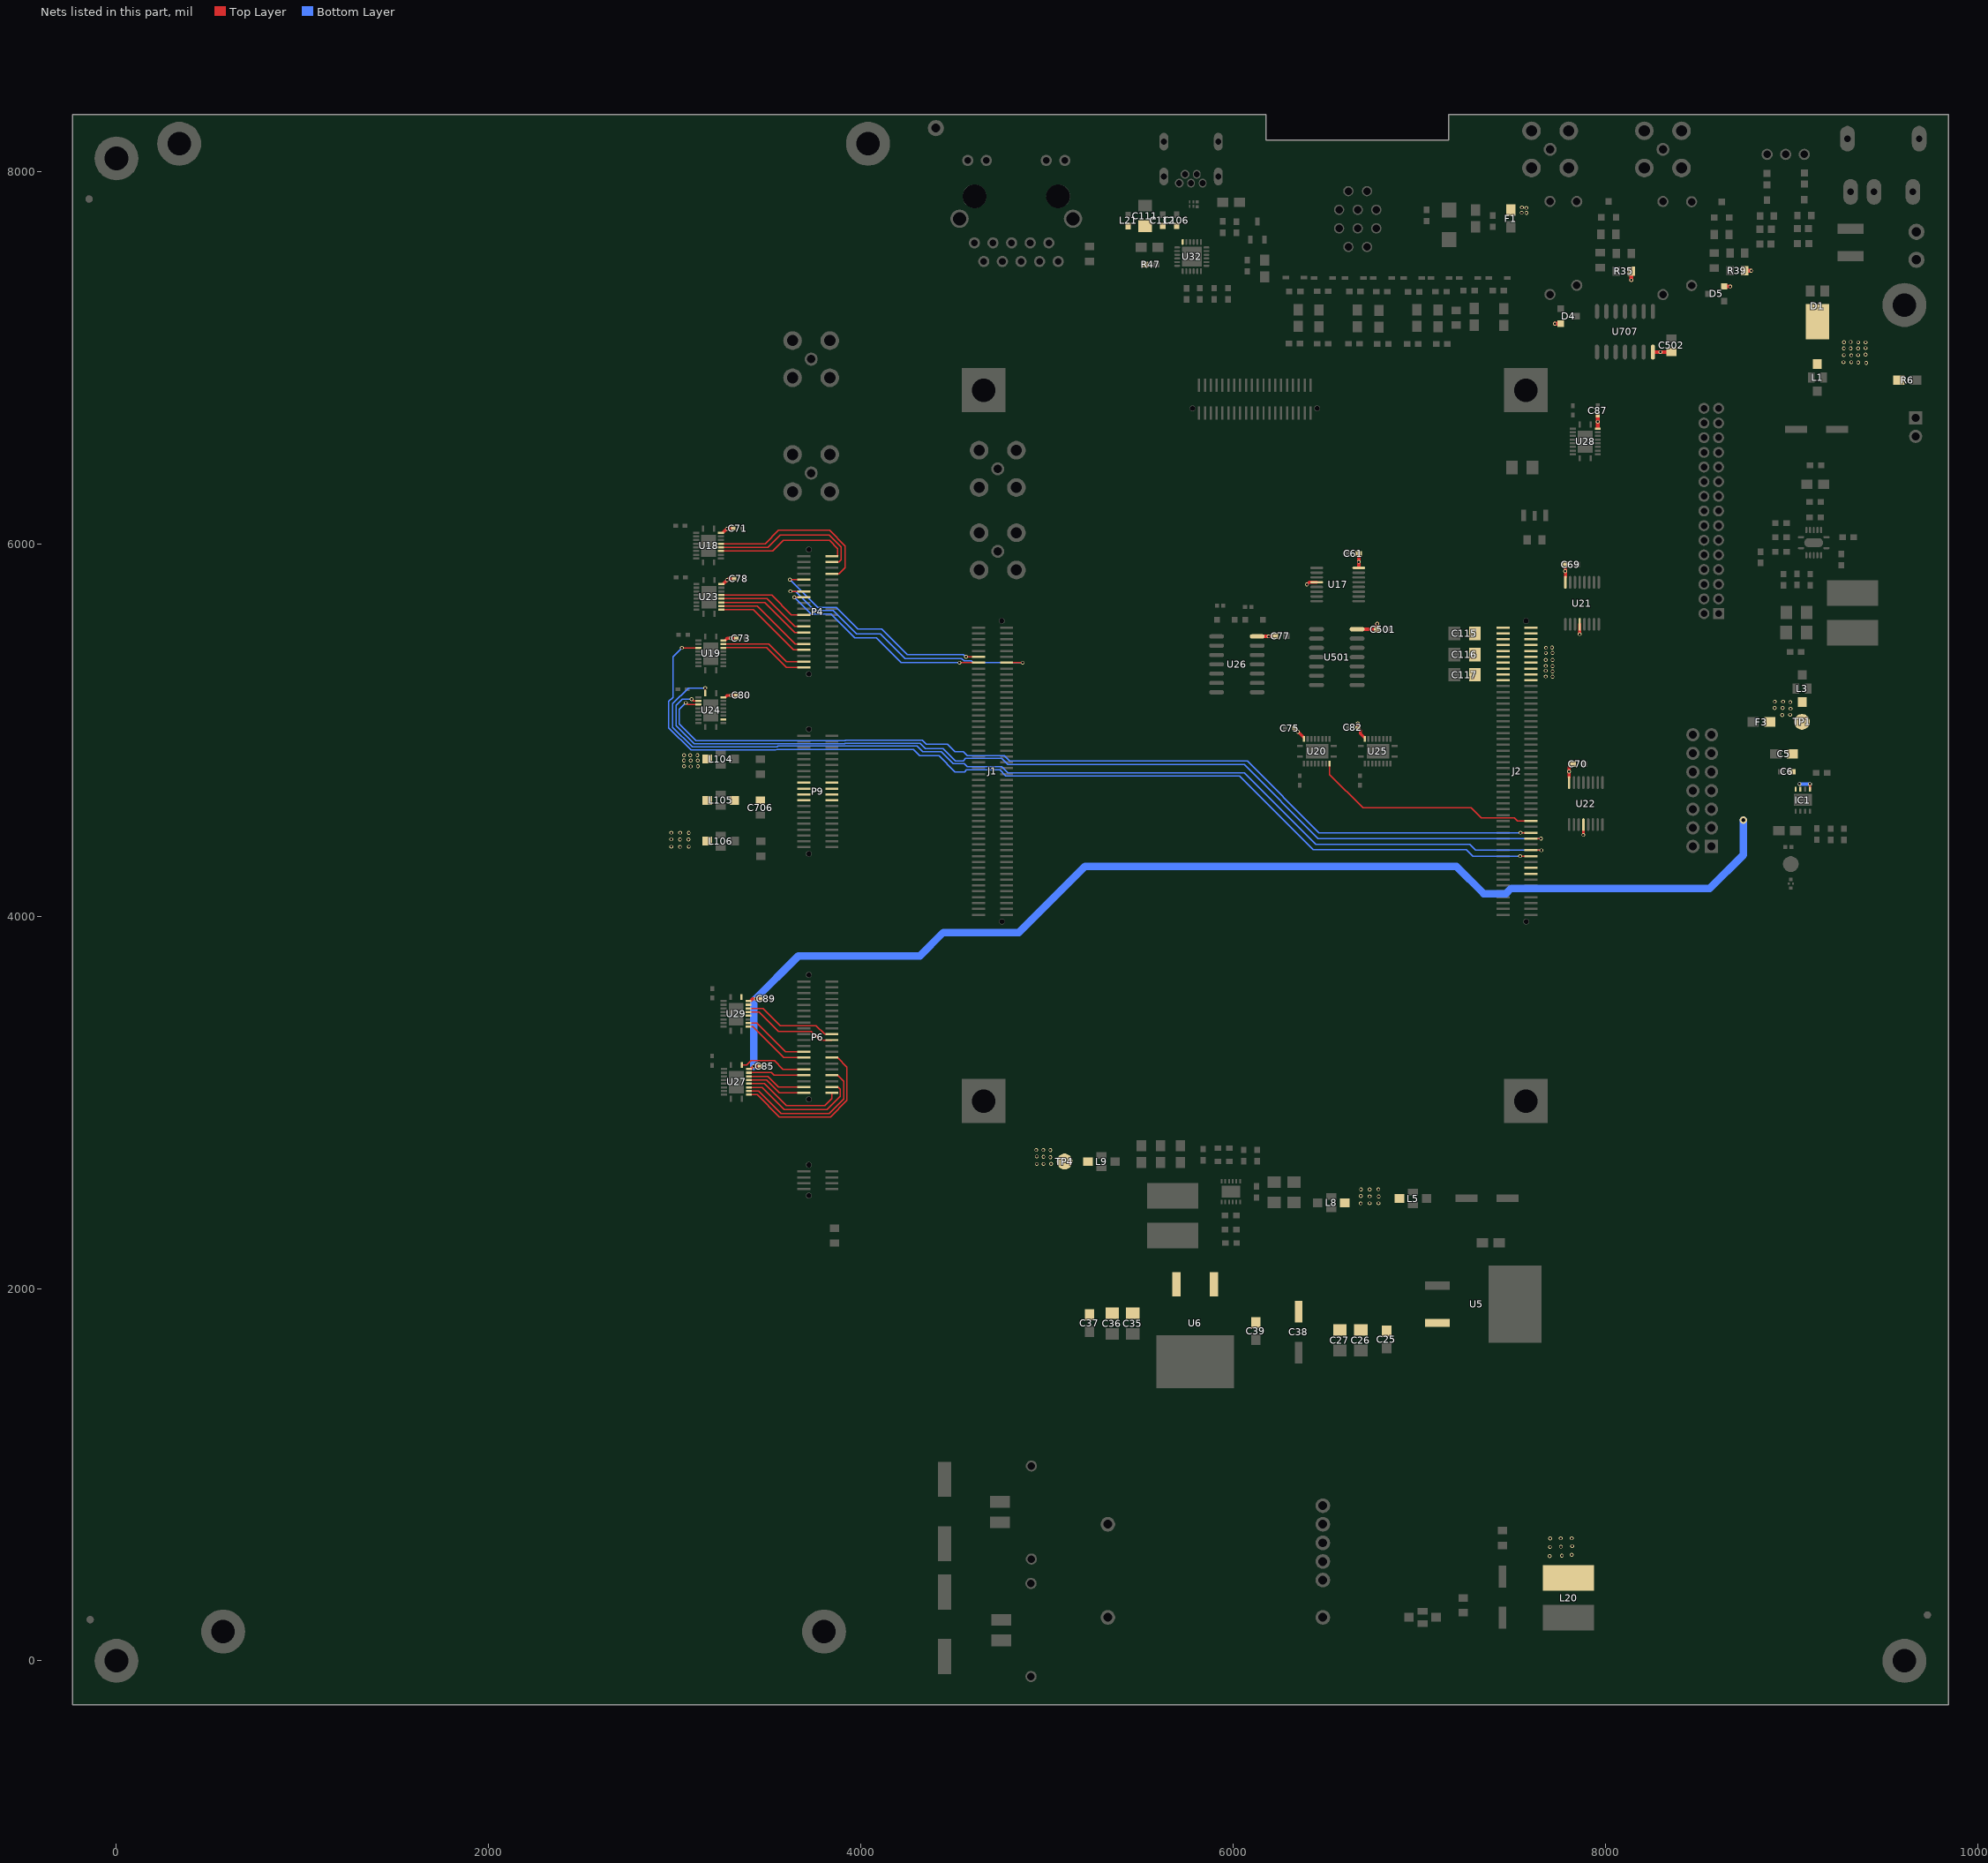
[diagram p0: the nets of this part, all layers, seen from the top]
# Altium PCB MISC82191.PcbDoc (part 4 of 9)
Units mil, origin at the board's own origin, x right, y up, seen from the top; angles counter-clockwise.
Board outline 10078.74 x 8543.31 mil, 4 copper layers (Top Layer, GND, POWER, Bottom Layer); 238 components, 299 nets, 1297 pads, 1665 vias.

## Via types
v1: diameter 20, hole 12, Top Layer to Bottom Layer, 1664 vias
v2: diameter 40, hole 20, Top Layer to Bottom Layer, 1 vias

## Nets (pads, with @x,y where several pads share a name; then routed paths per layer and width w, separated by ;. In a path a pad name is that pad's centre, name@x,y a point inside that pad or via, vN(x,y) a via of type N, cw(c..) or ccw(c..) an arc to the next point about the centre after c; other vN are vias at no path point) (continued)
3VIO58: J2.A34 U20.9 | length 1242
  Top Layer w6: U20.9@6518.25,4819.32 6518.25,4761.68 6697.78,4582.16 7277.78,4582.16 7331.78,4528.16 7509.78,4528.16 7526.3,4511.64 J2.A34@7599.01,4511.64
3VIO60: J2.A37 U24.3 | length 5298.9
  Top Layer w6: v1(3089.78,5166.16) 3099.5,5156.44 U24.3@3126.38,5156.44 ; J2.A37@7599.01,4417.15 v1(7653.79,4417.15)
  Bottom Layer w6: v1(3089.78,5166.16) 3040.78,5166.16 3007.78,5133.16 3007.78,5024.16 3104.53,4927.41 3912.03,4927.41 3913.78,4929.16 ; 3921.78,4929.16 3913.78,4929.16 ; 4907.78,4814.16 4900.78,4814.16 ; 7627.78,4417.16 7551.78,4417.16 ; v1@7652.78,4417.16 7551.78,4417.16 ; 3913.78,4929.16 4317.78,4929.16 4345.78,4901.16 4440.78,4901.16 4506.78,4835.16 4549.78,4835.16 4561.78,4847.16 4756.78,4847.16 4789.78,4814.16 4900.78,4814.16 ; 4900.78,4814.16 6059.03,4814.16 6456.03,4417.16 7551.78,4417.16
3VIO61: J2.A40 U19.4 | length 5542.8
  Top Layer w6: v1(3038.18,5441.76) U19.4@3126.38,5441.76 ; v1(7541.28,4322.66) J2.A40@7599.01,4322.66
  Bottom Layer w6: v1(3038.18,5441.76) 2989.78,5393.35 2989.78,5176.16 2966.78,5153.16 2966.78,5012.16 3086.53,4892.41 3543.03,4892.41 3546.78,4896.16 ; 3561.78,4896.16 3546.78,4896.16 ; 3881.53,4895.41 4282.78,4895.41 4316.03,4862.16 4342.78,4862.16 ; 3881.53,4896.16 3546.78,4896.16 ; 4320.78,4862.16 4342.78,4862.16 ; 4920.78,4753.16 4908.78,4753.16 ; 7518.78,4322.16 7499.78,4322.16 ; v1@7538.78,4322.16 7499.78,4322.16 ; 4342.78,4862.16 4418.78,4862.16 4505.78,4775.16 4556.78,4775.16 4567.78,4786.16 4745.78,4786.16 4778.78,4753.16 4908.78,4753.16 ; 4908.78,4753.16 6034.03,4753.16 6430.03,4357.16 7252.03,4357.16 7287.03,4322.16 7499.78,4322.16
3VIO62: J2.A39 U24.1 | length 5480.7
  Top Layer w6: U24.1@3163.78,5197.78 v1(3163.78,5226.16) ; J2.A39@7599.01,4354.16 v1(7655.78,4354.16)
  Bottom Layer w6: v1(3163.78,5226.16) 3073.78,5226.16 2988.78,5141.16 2988.78,5014.16 3093.53,4909.41 3549.03,4909.41 3553.78,4914.16 ; 3561.78,4914.16 3553.78,4914.16 ; 4920.78,4771.16 4911.78,4771.16 ; 7636.78,4355.16 7540.78,4355.16 ; v1@7656.78,4354.16 7655.78,4355.16 7540.78,4355.16 ; 3553.78,4914.16 4301.78,4914.16 4332.78,4883.16 4431.78,4883.16 4495.78,4819.16 4555.78,4819.16 4570.78,4804.16 4756.78,4804.16 4789.78,4771.16 4911.78,4771.16 ; 4911.78,4771.16 6060.03,4771.16 6444.03,4387.16 7271.03,4387.16 7303.03,4355.16 7540.78,4355.16
3VIO63: J2.A42
3VIO64: J2.A43
"9V 1.5A": C25.2 C26.2 C27.2 C38.1 C39.2 U5.3 U6.1
13V: C115.1 C116.2 C117.2 D1.3 J2.A1 J2.A2 J2.A3 J2.A4 J2.A5 J2.A6 J2.A7 J2.A8 J2.A9 J2.A10 J2.B1 J2.B2 J2.B3 J2.B4 J2.B5 J2.B6 J2.B7 J2.B8 J2.B9 J2.B10 L1.1 L5.1 L8.3 L20.1 L106.3 R6.1
  other v1: 7700.78,562.41 7765.78,565.41 7818.78,569.41 7701.78,611.41 7760.78,613.41 7820.78,616.41 7702.78,657.41 7759.78,658.41 7818.78,658.41 6684.78,2457.41 6732.78,2458.41 6780.78,2458.41 6781.78,2494.41 6732.78,2495.41 6685.78,2496.41 6686.78,2532.41 6732.78,2532.41 6779.78,2533.41 3027.78,4372.41 2980.78,4373.41 3074.78,4373.41 3027.78,4412.41 3073.78,4412.41 2980.78,4413.41 3074.78,4447.41 2980.78,4448.41 3028.78,4448.41 7715.78,5286.78 7678.78,5287.78 7715.78,5314.78 7678.78,5318.78 7715.78,5343.78 7678.78,5344.78 7678.78,5376.78 7715.78,5376.78 7679.78,5413.78 7715.78,5414.78 7680.78,5441.78 7712.78,5443.78 9400.78,6972.16 9357.78,6974.16 9278.78,6976.16 9320.78,6976.16 9320.78,7013.16 9280.78,7014.16 9356.78,7014.16 9397.78,7017.16 9280.78,7050.16 9317.78,7050.16 9356.78,7050.16 9397.78,7052.16 9357.78,7082.78 9397.78,7082.78 9281.78,7083.78 9317.78,7084.78
-5.4V: L9.3 L104.3 TP4.1
  other v1: 4944.78,2669.41 4980.78,2669.41 5021.78,2670.41 5017.78,2705.41 4980.78,2707.41 4944.78,2709.41 5017.78,2743.41 4941.78,2744.41 4979.78,2744.41 3084.78,4804.41 3049.78,4805.41 3123.78,4805.41 3048.78,4836.41 3084.78,4836.41 3122.78,4836.41 3082.78,4864.41 3121.78,4864.41 3049.78,4865.41
A6V: C35.2 C36.2 C37.2 L105.3 U6.3
A6V4: C706.2 L105.1 P9.17 P9.18 P9.19 P9.20 P9.21 P9.22 P9.23 P9.24
AK0: J2.A36 U24.4 | length 5040.2
  Top Layer w6: v1(3058.78,5146.16) 3068.18,5136.76 U24.4@3126.38,5136.76 ; v1(7544.29,4448.65) J2.A36@7599.01,4448.65
  Bottom Layer w6: v1(3058.78,5146.16) 3023.78,5111.16 3023.78,5032.16 3101.15,4954.78 3104.15,4951.78 3112.53,4943.41 3914.03,4943.41 3916.78,4946.16 ; 3932.78,4946.16 3916.78,4946.16 ; 4908.78,4834.16 4903.78,4834.16 ; v1(7544.29,4448.65) 6461.54,4448.65 6076.03,4834.16 4903.78,4834.16 ; 3916.78,4946.16 4328.78,4946.16 4350.78,4924.16 4464.78,4924.16 4504.78,4884.16 4549.78,4884.16 4570.78,4863.16 4769.78,4863.16 4798.78,4834.16 4903.78,4834.16
AK1: P6.28 U27.12 | length 883.7
  Top Layer w6: U27.12@3408.78,3041.16 3442.78,3041.16 3562.78,2921.16 3835.78,2921.16 3924.78,3010.16 3924.78,3189.16 3873.61,3240.33 P6.28@3843.82,3240.33
AK2: P6.34 U27.13 | length 754.2
  Top Layer w6: U27.13@3408.78,3061.16 3449.78,3061.16 3571.78,2939.16 3828.78,2939.16 3907.78,3018.16 3907.78,3112.16 3874.09,3145.84 P6.34@3843.82,3145.84
AK3: P6.37 U27.17 | length 438.3
  Top Layer w6: U27.17@3398.24,3139.76 3500.18,3139.76 3557.09,3082.85 P6.37@3694.21,3082.85 3575.47,3082.85
AK4: P6.38 U27.14 | length 659.1
  Top Layer w6: U27.14@3398.24,3080.7 3468.24,3080.7 3587.78,2961.16 3817.78,2961.16 3889.78,3033.16 3889.78,3070.16 3877.09,3082.85 P6.38@3843.82,3082.85
AK5: P6.39 U27.16 | length 443.2
  Top Layer w6: U27.16@3404.78,3120.16 3491.78,3120.16 3560.58,3051.35 P6.39@3694.21,3051.35 3568.98,3051.35
AK6: P6.33 U27.18 | length 357.3
  Top Layer w6: U27.18@3398.24,3159.44 3519.5,3159.44 3533.09,3145.84 3625.78,3145.84 ; 3570.09,3145.84 3625.78,3145.84 ; P6.33@3694.21,3145.84 3625.78,3145.84
AK7: P6.31 U27.20 | length 362.5
  Top Layer w6: U27.20@3360.83,3200.78 3386.4,3200.78 3409.78,3224.16 3534.78,3224.16 3581.6,3177.34 P6.31@3694.21,3177.34
AK8: P6.27 U29.12 | length 366.7
  Top Layer w6: U29.12@3396.24,3406.33 3419.61,3406.33 3585.61,3240.33 P6.27@3694.21,3240.33
AK9: P6.25 U29.13 | length 361.8
  Top Layer w6: U29.13@3396.24,3426.02 3439.92,3426.02 3594.11,3271.83 P6.25@3694.21,3271.83
AK10: P6.20 U29.17 | length 505
  Top Layer w6: U29.17@3396.24,3504.76 3474.18,3504.76 3566.22,3412.72 3759.22,3412.72 3805.78,3366.16 P6.20@3820.78,3366.16 ; P6.20@3820.78,3366.31 P6.20@3843.82,3366.31
AK11: U29.18
AK12: U29.15
AK13: P6.22 U29.16 | length 509.9
  Top Layer w6: U29.16@3396.24,3485.07 3452.87,3485.07 3556.78,3381.16 3654.99,3381.16 3655.05,3381.22 3733.37,3381.22 3779.77,3334.82 P6.22@3843.82,3334.82
AK16: U29.20
AS19: U24.13
AS20: P4.4 U18.15 | length 823.1
  Top Layer w6: U18.15@3248.14,5981.39 3500.01,5981.39 3565.78,6047.16 3829.78,6047.16 3893.78,5983.16 3893.78,5914.16 3882.39,5902.76 P4.4@3843.82,5902.76
AS23: P4.8 U18.16 | length 932.7
  Top Layer w6: U18.16@3248.14,6001.07 3485.69,6001.07 3557.78,6073.16 3830.78,6073.16 3914.78,5989.16 3914.78,5872.16 3882.39,5839.77 P4.8@3843.82,5839.77
AS24: P4.2 U18.14 | length 740.7
  Top Layer w6: U18.14@3248.14,5961.7 3526.32,5961.7 3582.78,6018.16 3830.78,6018.16 3874.78,5974.16 3874.78,5935.36 3875.88,5934.26 P4.2@3843.82,5934.26
AS27: P4.37 U19.18 | length 471.8
  Top Layer w6: U19.18@3266.78,5461.16 3290.78,5461.16 ; 3285.24,5461.16 3290.78,5461.16 ; P4.37@3694.21,5367.33 3598.61,5367.33 3504.78,5461.16 3290.78,5461.16
AS28: P4.39 U19.17 | length 479
  Top Layer w6: U19.17@3266.78,5442.16 3292.78,5442.16 ; 3285.24,5442.16 3292.78,5442.16 ; P4.39@3694.21,5335.83 3599.1,5335.83 3492.78,5442.16 3292.78,5442.16
ATTN1: P4.33 U23.12 | length 533.4
  Top Layer w6: U23.12@3250.24,5646.33 3421.61,5646.33 3637.61,5430.32 P4.33@3694.21,5430.32
ATTN2: P4.31 U23.13 | length 528.6
  Top Layer w6: U23.13@3250.24,5666.02 3443.92,5666.02 3648.12,5461.82 P4.31@3694.21,5461.82
ATTN4: P4.27 U23.14 | length 510.6
  Top Layer w6: U23.14@3250.24,5685.7 3483.24,5685.7 3644.13,5524.81 P4.27@3694.21,5524.81
ATTN8: P4.25 U23.15 | length 505.7
  Top Layer w6: U23.15@3250.24,5705.39 3494.55,5705.39 3643.63,5556.31 P4.25@3694.21,5556.31
ATTN16: P4.21 U23.16 | length 487.8
  Top Layer w6: U23.16@3250.24,5725.07 3520.87,5725.07 3626.64,5619.3 P4.21@3694.21,5619.3
C3.3V: C106.2 C111.1 C112.1 L21.1 R47.2 U32.6
D5V: C5.2 C6.2 C61.2 C69.2 C70.2 C71.1 C73.1 C75.1 C77.2 C78.1 C80.1 C82.1 C85.1 C87.1 C89.1 C501.2 C502.2 D4.2 D5.2 F1.2 F3.2 IC1.5 IC1.7 IC1.8 L3.3 R35.2 R39.2 TP1.1 U17.4 U17.16 U18.19 U19.19 U20.19 U21.4 U21.16 U22.4 U22.16 U23.19 U24.19 U25.19 U26.14 U27.19 U28.19 U29.19 U501.14 U707.14 | length 7821.9
  Top Layer w11: IC1.5@9098.55,4681.31 v1(9098.55,4709.93)
  Top Layer w16: U18.19@3260.78,6063.16 v1@3280.78,6083.16 ; U23.19@3261.78,5787.16 v1(3280.78,5806.16) 3287.78,5813.16 C78.1@3318.78,5813.16 ; U19.19@3271.78,5484.16 3280.78,5493.16 v1@3301.78,5493.16 ; U24.19@3274.78,5179.16 3281.78,5186.16 v1(3302.78,5186.16) C80.1@3331.78,5186.16 ; v1(3280.78,6081.16) v1@3280.78,6083.16 ; v1(3300.78,5493.16) v1@3301.78,5493.16 ; C71.1@3313.78,6083.16 v1@3280.78,6083.16 ; C73.1@3330.78,5493.16 v1@3301.78,5493.16 ; U29.19@3408.78,3547.16 3417.78,3556.16 v1@3434.78,3556.16 ; U27.19@3409.78,3182.16 3421.78,3194.16 v1(3424.78,3194.16) C85.1@3457.78,3194.16 ; v1(3435.78,3556.16) C89.1@3464.78,3556.16 ; C75.1@6329.78,5009.16 v1@6348.28,4990.66 ; v1(6347.78,4990.16) v1@6348.28,4990.66 ; U20.19@6376.78,4962.16 v1@6348.28,4990.66 ; v1(6395.78,5782.16) 6408,5794.38 U17.4@6448.78,5794.38 ; v1(6668.78,5036.16) C82.1@6668.78,5013.16 6683.78,4998.16 6683.78,4980.16 U25.19@6701.78,4962.16 ; v1(7783.78,5853.16) v1@7784.78,5853.16 ; U21.16@7784.78,5821.16 v1@7784.78,5853.16 ; C69.2@7784.78,5888.16 v1@7784.78,5853.16 ; U22.16@7804.78,4747.16 v1(7804.78,4777.16) 7804.78,4800.16 C70.2@7822.78,4818.16 ; v1(7861.56,5515.38) U21.4@7861.56,5568.16 ; v1(7881.56,4436.94) U22.4@7881.56,4492.16
  Top Layer w20: U26.14@6128.82,5503.16 v1(6189.78,5503.16) C77.2@6223.78,5503.16 ; U501.14@6665.7,5541.72 C501.2@6764.21,5541.72 ; U17.16@6674.78,5875.16 v1(6674.78,5904.16) C61.2@6674.78,5947.16 ; C501.2@6773.78,5541.16 v1(6773.78,5571.16) ; v1(7727.78,7183.16) D4.2@7759.78,7183.16 ; 7958.78,6626.16 v1(7958.78,6656.16) C87.1@7958.78,6692.16 ; v1(8138.78,7417.16) R35.2@8138.78,7464.16 ; U707.14@8261.78,7030.78 v1@8293.78,7030.78 ; v1(8295.78,7030.78) v1@8293.78,7030.78 ; C502.2@8354.78,7030.78 v1@8293.78,7030.78 ; D5.2@8637.78,7383.16 v1(8670.78,7383.16) ; R39.2@8748.78,7467.16 v1(8782.78,7467.16)
  Bottom Layer w20: v1(9042.55,4709.93) v1(9098.55,4709.93)
  Bottom Layer w40: v1(3424.78,3194.16) 3424.78,3547.41 3663.78,3786.41 4316.78,3786.41 4442.78,3912.41 4848.78,3912.41 5203.78,4267.41 7199.78,4267.41 7345.78,4121.41 7465.78,4121.41 7493.78,4149.41 8560.78,4149.41 8740.78,4329.41 v2(8740.78,4516.41)
  other v1: 8949.78,5080.41 8991.78,5082.41 8994.78,5114.41 8908.78,5118.41 8951.78,5118.41 8992.78,5150.41 8909.78,5152.41 8953.78,5152.41 7575.78,7778.16 7549.78,7779.16 7574.78,7805.16 7550.78,7807.16
"DAC CLK": J1.A7 P4.13 | length 1566.7
  Top Layer w6: v1(3620.91,5745.28) P4.13@3694.21,5745.28 ; J1.A7@4782.37,5362.01 v1(4868.93,5362.01)
  Bottom Layer w6: v1(3620.91,5745.28) 3648.65,5745.28 3751.78,5642.16 3851.03,5642.16 3975.78,5517.41 4103.78,5517.41 4236.03,5385.16 4540.78,5385.16 4554.78,5371.16 4592.78,5371.16 4601.93,5362.01 v1(4868.93,5362.01)
"DAC DATA": J1.B7 P4.15 | length 1188.4
  Top Layer w6: v1(3642.15,5713.79) P4.15@3694.21,5713.79 ; v1(4529.63,5362.01) J1.B7@4632.75,5362.01
  Bottom Layer w6: v1(3642.15,5713.79) 3732.78,5623.16 3838.03,5623.16 3966.78,5494.41 4083.78,5494.41 4216.03,5362.16 4529.48,5362.16 v1(4529.63,5362.01)
"DAC STROBE": J1.B6 P4.9 | length 1258.9
  Top Layer w6: v1(3618.66,5808.28) P4.9@3694.21,5808.28 ; v1(4564.44,5393.5) J1.B6@4632.75,5393.5
  Bottom Layer w6: v1(3618.66,5808.28) 3766.78,5660.16 3867.78,5660.16 3984.53,5543.41 4111.78,5543.41 4250.03,5405.16 4549.78,5405.16 v1@4561.78,5393.16
DATA_T: P6.40 U27.15 | length 541.5
  Top Layer w6: U27.15@3398.24,3100.39 3481.55,3100.39 3599.78,2982.16 3805.78,2982.16 3843.82,3020.2 P6.40@3843.82,3051.35